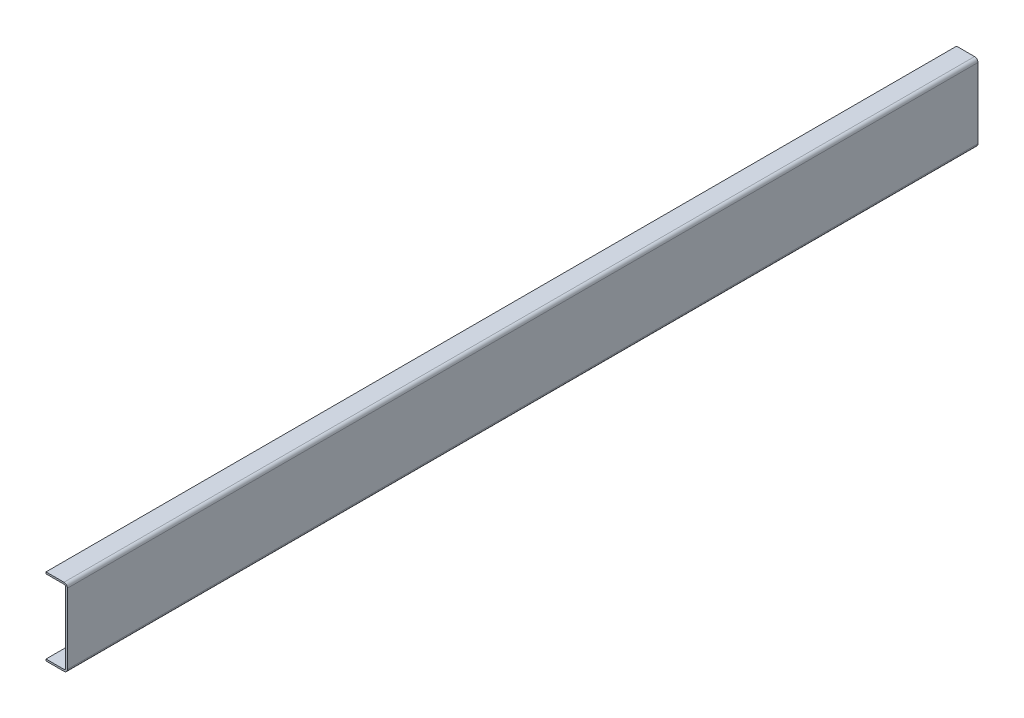
SolidWorks part; units mm, degrees
ref_plane "Front Plane" through (0, 0, 0) normal (0, 0, 1) x (1, 0, 0)
ref_plane "Top Plane" through (0, 0, 0) normal (0, 1, 0) x (1, 0, 0)
ref_plane "Right Plane" through (0, 0, 0) normal (1, 0, 0) x (0, 0, -1)
other "Configuration Table"
sketch "Sketch1" plane through (0, 0, 0) normal (0, 0, 1) x (1, 0, 0)
  line L0 (-50, -90) -> (-8, -90)
  line L1 (0, -82) -> (0, 82)
  line L2 (-8, 90) -> (-50, 90)
  line L3 (-50, 90) -> (-50, 86)
  line L4 (-50, 86) -> (-8, 86)
  line L5 (-4, 82) -> (-4, -82)
  line L6 (-8, -86) -> (-50, -86)
  line L7 (-50, -86) -> (-50, -90)
  arc A0 (-8, -90) -> (0, -82) centre (-8, -82) ccw
  arc A1 (0, 82) -> (-8, 90) centre (-8, 82) ccw
  arc A2 (-4, 82) -> (-8, 86) centre (-8, 82) ccw
  arc A3 (-8, -86) -> (-4, -82) centre (-8, -82) ccw
  dimension "D1" = 8
  dimension "D2" = 4
  dimension "D3" = 50
  dimension "D4" = 86
  dimension "D5" = 86
extrude "Boss-Extrude1" add sketch "Sketch1" along normal mid plane 2124
